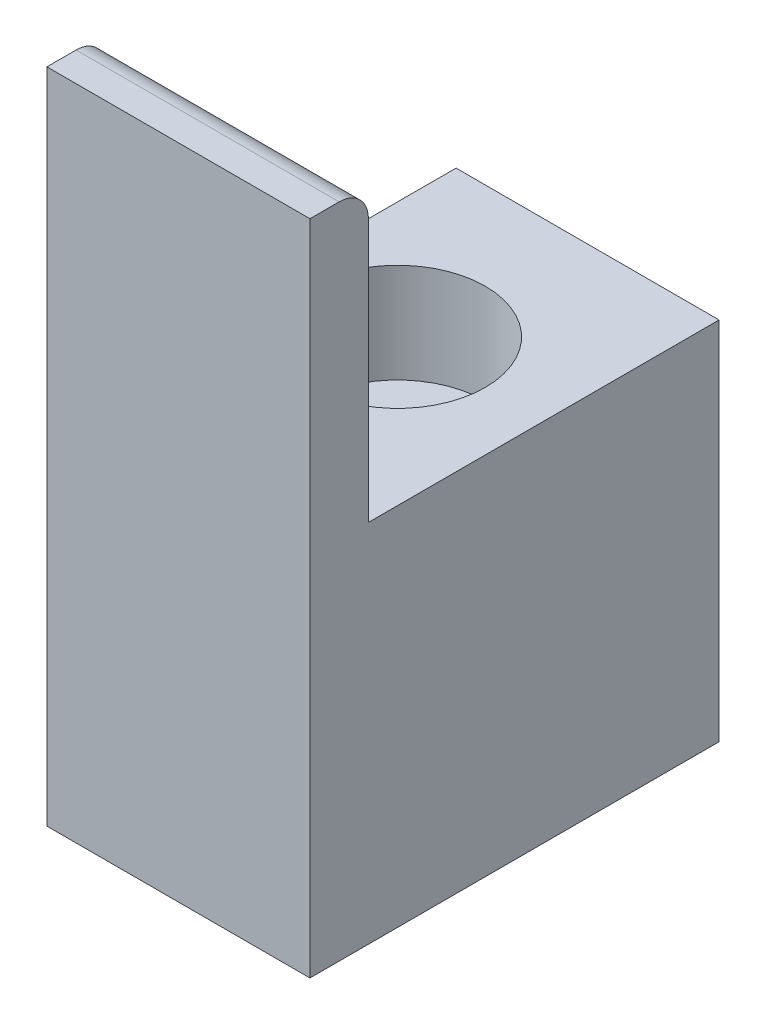
from build123d import *

# Parameters (mm, degrees)
SKETCH1_W                                         = 9
SKETCH1_H                                         = 14
BOSS_EXTRUDE1_DEPTH                               = 12.5
CUT_EXTRUDE1_DEPTH                                = 3
SKETCH3_W                                         = 9
SKETCH3_H                                         = 10
BOSS_EXTRUDE2_DEPTH                               = 2
FILLET1_R                                         = 1
HOLE_SIZE_PER_HEX_SOCKET_SCREW_TYPE_1_D           = 3.4
HOLE_SIZE_PER_HEX_SOCKET_SCREW_TYPE_1_CBORE_D     = 6
HOLE_SIZE_PER_HEX_SOCKET_SCREW_TYPE_1_CBORE_DEPTH = 3.4


with BuildPart() as part:
    # Sketch1 → Boss-Extrude1 (new body)
    with BuildSketch(Plane(origin=(0, 0, 0), x_dir=(1, 0, 0), z_dir=(0, 1, 0))):
        Rectangle(SKETCH1_W, SKETCH1_H)
    extrude(amount=BOSS_EXTRUDE1_DEPTH)

    # Sketch2 → Cut-Extrude1 (cut)
    with BuildSketch(Plane.XZ):
        with BuildLine():
            Line((1, 1), (-2, 1))
            ThreePointArc((-2, 1), (-3, -1), (-2, -3))
            Line((-2, -3), (1, -3))
            ThreePointArc((1, -3), (2, -1), (1, 1))
        make_face()
    extrude(amount=-CUT_EXTRUDE1_DEPTH, mode=Mode.SUBTRACT)

    # Sketch3 → Boss-Extrude2 (add)
    with BuildSketch(Plane.XY.offset(7)):
        with Locations((0, 17.5)):
            Rectangle(SKETCH3_W, SKETCH3_H)
    extrude(amount=-BOSS_EXTRUDE2_DEPTH)

    # Fillet1
    fillet1_edges = [part.edges().sort_by_distance(p)[0] for p in [
        (0, 22.5, 5),
    ]]
    fillet(fillet1_edges, radius=FILLET1_R)

    # Hole size (per hex socket screw type) 1 (through all)
    with Locations(Plane(origin=(-0.5, 12.5, -1), x_dir=(0, 0, 1), z_dir=(0, 1, 0))):
        with Locations((0, 0)):
            CounterBoreHole(HOLE_SIZE_PER_HEX_SOCKET_SCREW_TYPE_1_D / 2, HOLE_SIZE_PER_HEX_SOCKET_SCREW_TYPE_1_CBORE_D / 2, HOLE_SIZE_PER_HEX_SOCKET_SCREW_TYPE_1_CBORE_DEPTH)


solid = part.part
